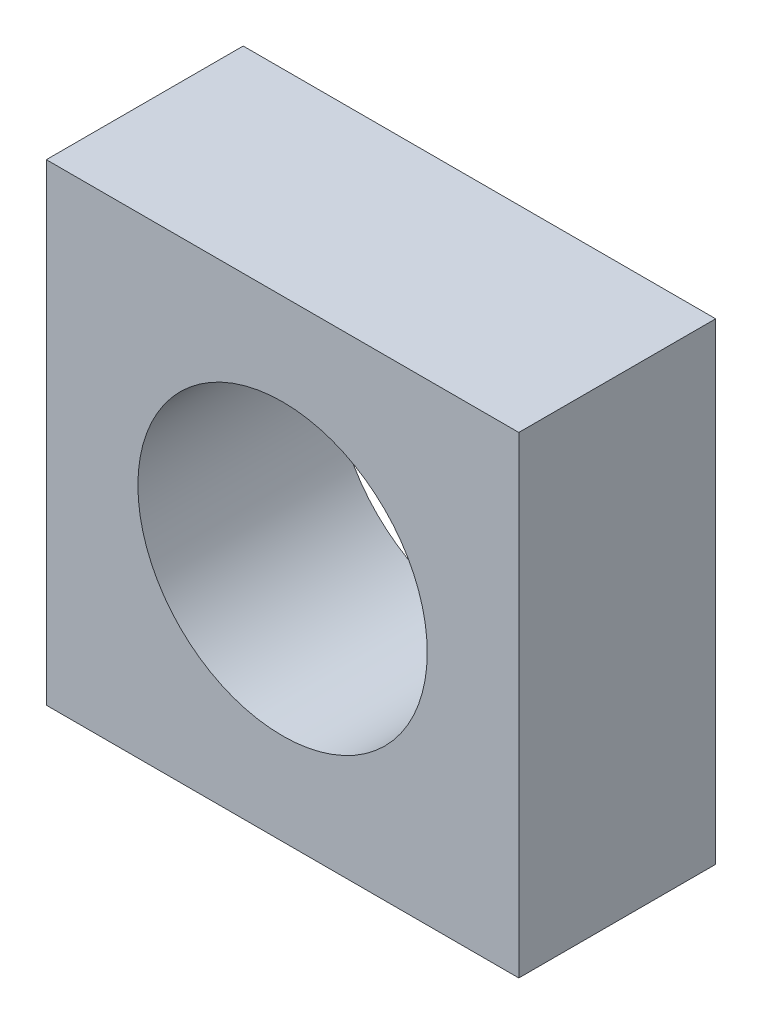
SolidWorks part; units mm, degrees
ref_plane "Front Plane" through (0, 0, 0) normal (0, 0, 1) x (1, 0, 0)
ref_plane "Top Plane" through (0, 0, 0) normal (0, 1, 0) x (1, 0, 0)
ref_plane "Right Plane" through (0, 0, 0) normal (1, 0, 0) x (0, 0, -1)
other "Configuration Table"
sketch "Sketch1" plane through (0, 0, 0) normal (0, 0, 1) x (1, 0, 0)
  line L1 (-33.0657, 6) -> (-21.0657, 6)
  line L2 (-33.0657, 6) -> (-33.0657, -6)
  line L3 (-33.0657, -6) -> (-21.0657, -6)
  line L4 (-21.0657, 6) -> (-21.0657, -6)
  line L5 (-33.0657, 6) -> (-21.0657, -6) construction
  line L6 (-33.0657, -6) -> (-21.0657, 6) construction
  circle A2 centre (-27.0657, 0) radius 3.6746
  point P0 (-27.0657, 0)
extrude "Boss-Extrude1" add sketch "Sketch1" against normal blind 5
